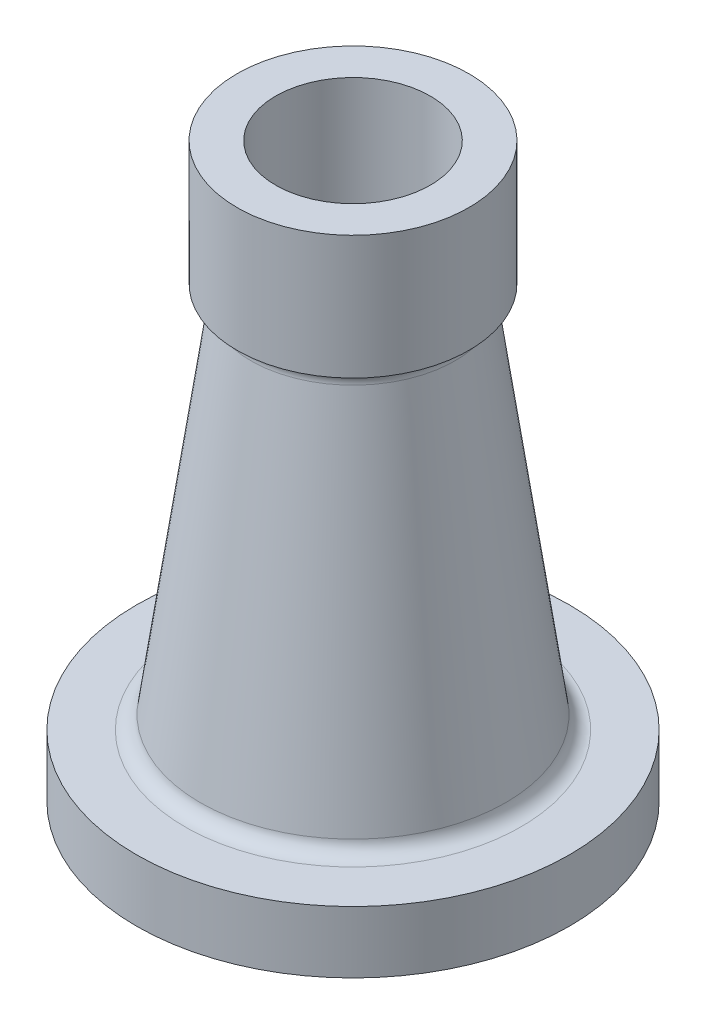
from build123d import *


with BuildPart() as part:
    # Sketch1 → Revolve1 (revolve)
    with BuildSketch(Plane.XY, mode=Mode.PRIVATE) as revolve1_sk:
        with BuildLine():
            Line((37.5, 92.5), (25, 92.5))
            Line((25, 92.5), (25, 25.700367412))
            Line((25, 25.700367412), (41.295159506, -89.5))
            Line((41.295159506, -89.5), (50, -89.5))
            Line((50, -89.5), (50, -92.5))
            Line((50, -92.5), (70, -92.5))
            Line((70, -92.5), (70, -72.5))
            Line((70, -72.5), (54.342520005, -72.5))
            ThreePointArc((54.342520005, -72.5), (51.063908223, -71.275010567), (49.391802356, -68.200281914))
            Line((49.391802356, -68.200281914), (33.044354116, 47.369746278))
            ThreePointArc((33.044354116, 47.369746278), (34.102490489, 50.950750604), (37.5, 52.5))
            Line((37.5, 52.5), (37.5, 92.5))
        make_face()
    revolve(revolve1_sk.sketch.rotate(Axis((0, 92.5, 0), (0, -1, 0)), 180), axis=Axis((0, 92.5, 0), (0, -1, 0)))


solid = part.part
